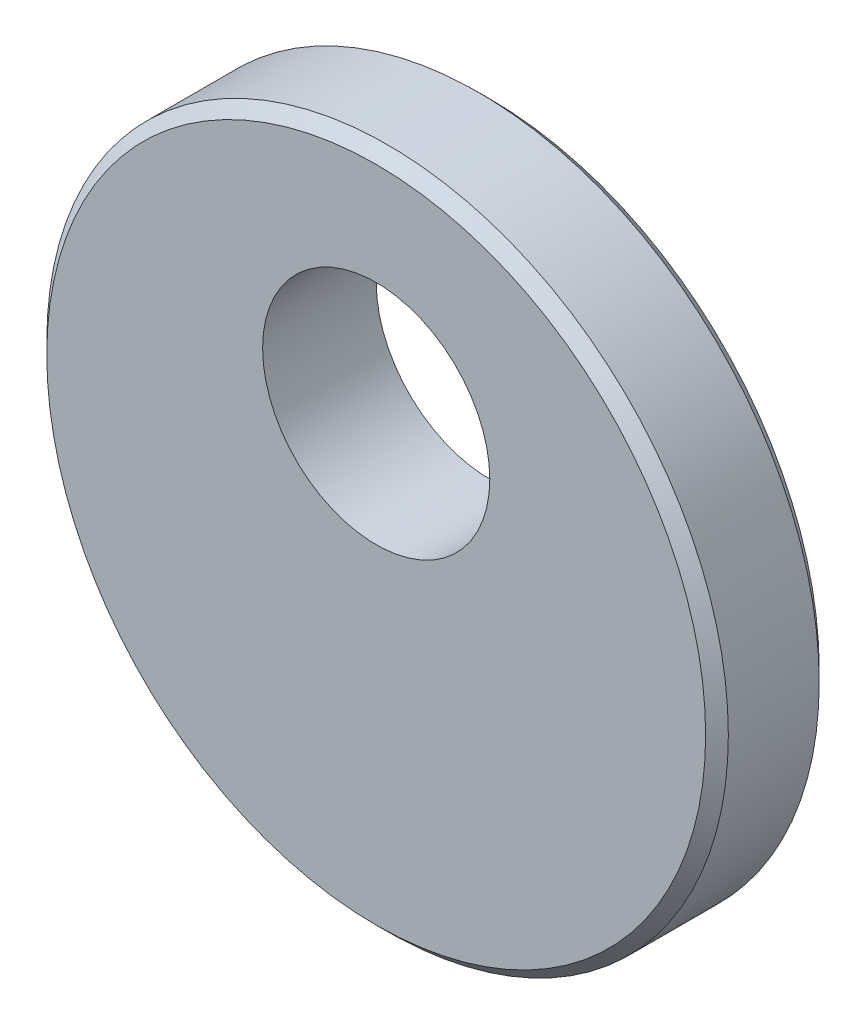
SolidWorks part; units mm, degrees
ref_plane "Front Plane" through (0, 0, 0) normal (0, 0, 1) x (1, 0, 0)
ref_plane "Top Plane" through (0, 0, 0) normal (0, 1, 0) x (1, 0, 0)
ref_plane "Right Plane" through (0, 0, 0) normal (1, 0, 0) x (0, 0, -1)
other "Configuration Table"
sketch "Sketch1" plane through (0, 0, 0) normal (0, 0, 1) x (1, 0, 0)
  circle A0 centre (0, 0) radius 15
  dimension "D1" = 30
extrude "Boss-Extrude1" add sketch "Sketch1" along normal blind 5
sketch "Sketch2" plane through (0, 0, 5) normal (0, 0, 1) x (1, 0, 0)
  line L0 (0, 5) -> (0, 0) construction
  line L1 (-4.894, 0) -> (8.7989, 0) construction
  circle A0 centre (0, 5) radius 5
  dimension "D1" = 5
extrude "Cut-Extrude1" cut sketch "Sketch2" against normal blind 5
chamfer "Chamfer1" distance 0.5 angle 45 2 edges at (15, 0, 0) (15, 0, 5)
